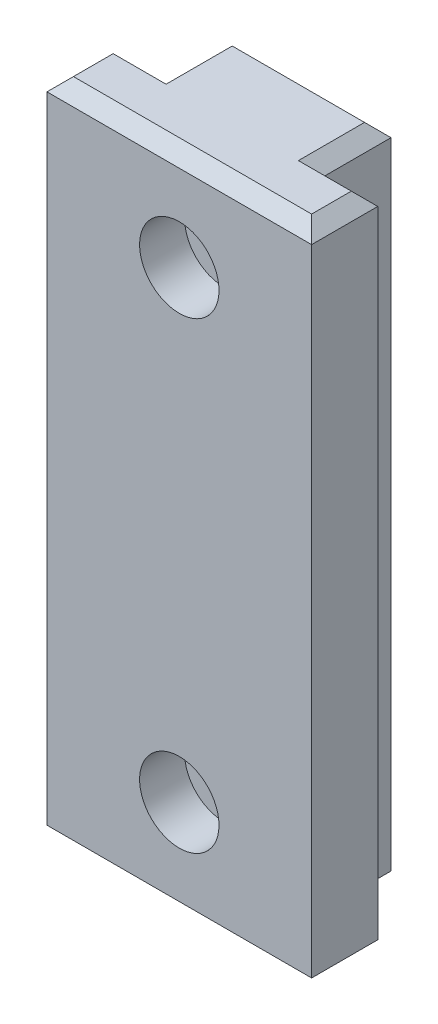
from build123d import *

# Parameters (mm, degrees)
EXTRUDE_1_DEPTH              = 50
CHAMFER_1_SIZE               = 1
HOLE_WIZARD_M3_1_D           = 3.4
HOLE_WIZARD_M3_1_CBORE_D     = 6
HOLE_WIZARD_M3_1_CBORE_DEPTH = 3.4


with BuildPart() as part:
    # 草图1 → 凸台-拉伸1 (new body)
    with BuildSketch(Plane(origin=(0, 0, 0), x_dir=(1, 0, 0), z_dir=(0, 1, 0))):
        Polygon((10, 0), (-10, 0), (-10, 5), (-6, 5), (-6, 10), (6, 10), (6, 5), (10, 5), align=None)
    extrude(amount=EXTRUDE_1_DEPTH)

    # 倒角1
    chamfer_1_edges = [part.edges().sort_by_distance(p)[0] for p in [
        (8, 0, -5),
        (10, 0, -2.5),
        (0, 0, 0),
        (-10, 0, -2.5),
        (10, 50, -2.5),
        (8, 50, -5),
        (6, 50, -7.5),
        (0, 50, -10),
        (-6, 50, -7.5),
        (-8, 50, -5),
        (-10, 50, -2.5),
        (-8, 0, -5),
        (0, 50, 0),
        (-6, 0, -7.5),
        (0, 0, -10),
        (6, 0, -7.5),
    ]]
    chamfer(chamfer_1_edges, length=CHAMFER_1_SIZE)

    # M3 六角圆柱头螺钉的柱形沉头孔1 (through all)
    with Locations(Plane.XY):
        with Locations((0, 42.5), (0, 7.5)):
            CounterBoreHole(HOLE_WIZARD_M3_1_D / 2, HOLE_WIZARD_M3_1_CBORE_D / 2, HOLE_WIZARD_M3_1_CBORE_DEPTH)


solid = part.part
